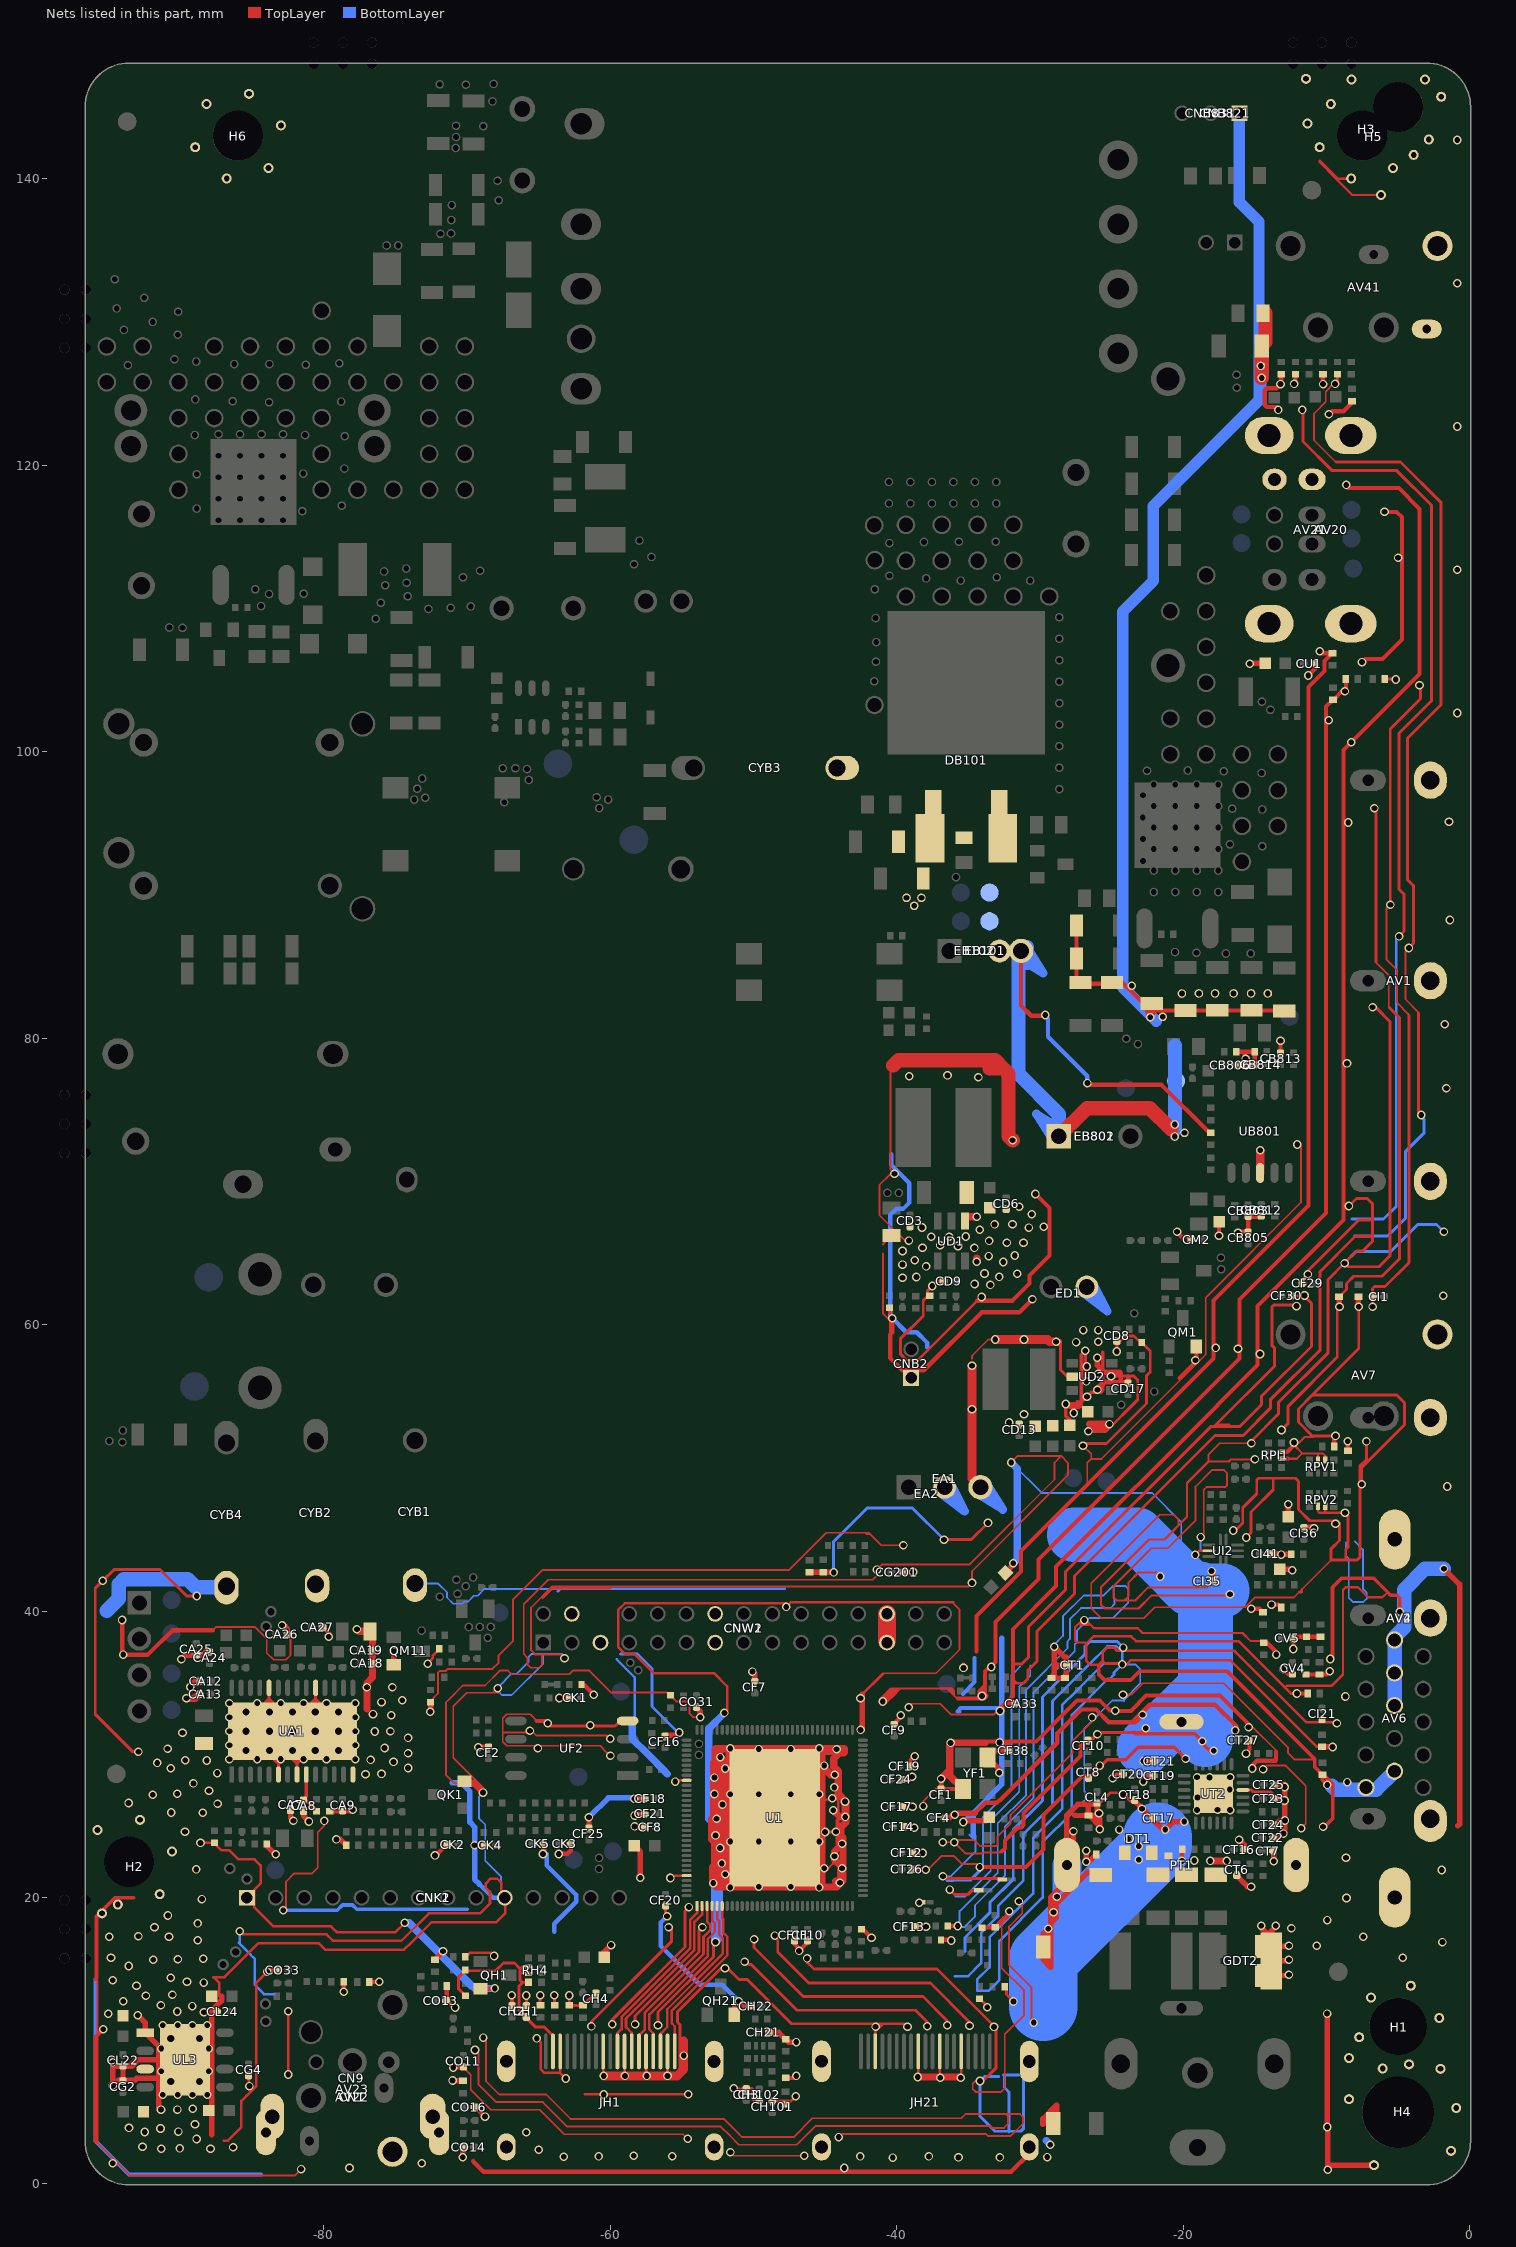
[diagram p0: the nets of this part, all layers, seen from the top]
# Altium PCB MISC86372.PcbDoc (part 10 of 16)
Units mm, origin at the board's own origin, x right, y up, seen from the top; angles counter-clockwise.
Board outline 96.73 x 148.13 mm, 2 copper layers (TopLayer, BottomLayer), stack 1.571 mm thick; 578 components, 318 nets, 2702 pads, 836 vias.

## Via types
v1: diameter 0.6, hole 0.4, TopLayer to BottomLayer, tented both sides, 816 vias
v2: diameter 0.7, hole 0.5, TopLayer to BottomLayer, tented both sides, 15 vias
v3: diameter 0.8, hole 0.5, TopLayer to BottomLayer, tented both sides, 5 vias

## Nets (pads, with @x,y where several pads share a name; then routed paths per layer and width w, separated by ;. In a path a pad name is that pad's centre, name@x,y a point inside that pad or via, vN(x,y) a via of type N, cw(c..) or ccw(c..) an arc to the next point about the centre after c; other vN are vias at no path point) (continued)
GND: (continued)
  TopLayer w0.381: CL22.2@-94.018,8.215 -94.018,7.235 CG2.1@-94.027,7.227 ; v1(-92.989,11.786) -92.471,11.267 UL3.1@-92.471,10.565 -91.535,9.628 -91.535,9.068 ; v1(-91.362,5.193) -91.535,5.365 -91.535,9.068 ; v1(-91.342,9.451) -91.535,9.258 -91.535,9.068 ; v1(-89.941,36.636) -89.664,36.913 -88.519,36.913 -88.255,37.176 CA24.1@-87.979,37.176 ; -87.817,3.445 -87.817,12.148 -87.252,12.713 -87.227,12.713 -87.114,12.826 -87.114,13.106 ; RA9.1@-83.972,23.724 -83.972,23.665 RA9.1@-83.917,23.61 ; RA9.1@-83.956,23.606 v1(-83.363,23.012) ; RA9.1@-83.917,23.568 RA9.1@-83.917,23.61 ; RA9.1@-83.917,23.728 RA9.1@-83.917,23.61 ; CA7.1@-82.324,26.043 -82.324,25.569 v1(-82.12,25.366) ; CA8.1@-81.417,25.981 -81.417,25.685 v1(-81.04,25.309) ; v1(-79.121,24.054) -78.841,24.054 DK1.A@-78.435,23.648 ; v1(-75.133,37.177) -75.108,37.151 QM11.E@-75.108,36.258 ; v1(-72.563,32.959) -72.542,32.98 RM12.2@-72.542,33.636 ; DO1.A@-72.238,15.665 -71.681,16.222 v1(-71.681,16.248) ; v1(-71.011,7.225) -70.979,7.193 DI8.A@-70.275,7.193 ; CO14.1@-70.312,2.577 -70.312,1.87 v1(-70.307,1.865) ; v1(-69.472,23.64) -69.462,23.63 CK4.2@-68.795,23.63 ; v1(-64.694,23.038) -64.631,23.1 CK5.2@-64.631,23.752 ; v1(-63.551,33.925) -63.535,33.941 CK1.1@-62.864,33.941 ; v1(-61.493,25.603) -61.487,25.597 CF25.2@-61.487,24.86 ; CF5.1@-60.406,15.824 -60.406,16.213 v1(-59.943,16.677) ; CF3.1@-58.321,23.628 -57.906,23.213 v1(-57.906,21.387) ; v1@-58.318,25.806 -57.651,25.806 CF21.2@-57.626,25.832 ; v1(-58.318,26.899) v1(-58.318,26.899) CF18.2@-57.634,26.898 ; v1@-58.318,26.924 -58.317,26.923 CF18.2@-57.634,26.923 ; -57.949,24.964 v1(-58.304,24.964) -58.28,24.94 CF8.1@-57.627,24.94 ; CF16.1@-56.185,31.286 -56.144,31.326 -55.389,31.326 v1(-55.194,31.521) ; CO31.1@-53.975,33.256 -53.722,33.002 v1(-53.722,32.578) ; v1(-50.076,35.773) -49.911,35.608 CF7.1@-49.911,35.096 ; CH21.2@-48.888,10.59 -48.24,10.59 DH23.A@-47.752,10.102 -47.556,9.906 v1(-47.015,9.906) ; CD101.A@-46.096,42.695 -45.156,42.695 CD102.A@-45.131,42.72 -44.428,42.72 v1(-44.403,42.696) ; v1(-42.524,31.699) -42.425,31.798 -42.425,33.807 v1(-42.534,33.916) -42.425,34.026 v1@-42.425,34.181 ; CF24.2@-39.605,28.245 -39.106,28.245 v1(-38.928,28.422) ; CG201.2@-39.58,42.723 v1@-38.862,42.723 ; CF14.1@-39.451,24.942 -38.843,24.942 v1(-38.773,24.872) ; CF13.1@-38.69,17.975 -37.985,17.975 v1(-37.959,17.95) ; CF4.1@-36.634,25.552 -36.304,25.552 ; CF4.1@-36.532,25.552 -36.304,25.552 ; v1(-35.956,25.786) v1@-36.07,25.786 ; v1@-35.325,25.241 v1(-35.357,25.273) -35.287,25.343 -33.802,25.343 CL3.1@-33.55,25.595 ; -34.533,25.895 -35.745,25.895 -35.855,25.786 v1@-36.07,25.786 ; YF1.4@-33.669,29.548 YF1.4@-33.669,29.777 ; v1@-32.919,28.778 v1(-32.842,28.702) -32.842,28.95 YF1.4@-33.669,29.777 ; CF15.1@-32.419,42.663 -31.877,43.205 v1(-31.877,43.332) ; -32.258,30.848 -32.258,30.391 -32.398,30.251 -33.194,30.251 YF1.4@-33.669,29.777 ; -29.413,15.596 CT47.1@-29.77,15.953 ; CT48.1@-29.084,4.208 -28.846,4.446 -28.846,5.498 -29.803,4.541 -29.803,4.166 -28.999,4.97 -28.999,5.135 ; -29.061,18.658 v1(-29.061,18.975) ; -29.007,36.22 CT1.2@-28.162,36.22 ; v1@-28.854,20.066 -29.061,19.859 -29.061,19.82 ; v1(-28.821,20.06) -29.061,19.82 ; -28.162,36.666 v1(-28.999,37.503) -29.007,37.495 -29.007,35.528 DK3.A@-29.21,35.325 DK2.A@-28.245,35.325 -28.162,35.407 -28.162,36.767 ; v1(-27.666,24.621) -27.666,22.719 PT1.4@-28.117,22.268 ; -27.559,25.756 -27.527,25.723 LT3.2@-26.619,25.723 ; v1(-26.764,23.256) v1(-26.764,22.498) -26.593,22.498 LT2.2@-26.079,23.012 ; -26.715,21.768 -26.715,21.721 -28.853,19.582 -28.853,18.593 -29.261,18.185 ; -26.619,26.51 LT3.2@-26.619,25.723 ; LT3.2@-26.556,25.723 -25.832,24.999 v1(-25.832,24.765) ; v1(-26.008,57.678) -26.008,57.162 -25.619,56.772 -25.522,56.675 -24.436,56.675 ; v1@-25.99,55.488 -25.99,55.542 -25.619,55.913 -25.522,56.01 ; CT18.2@-23.393,26.753 -22.885,26.245 v1(-22.885,26.187) -22.797,26.187 CT17.1@-22.142,25.532 -22.142,25.458 -21.423,24.74 -21.226,24.74 -20.667,25.298 v1(-19.939,25.298) ; DT1.3@-22.187,23.114 DT1.3@-22.187,23.177 ; CT6.1@-16.259,21.525 -16.259,21.49 -15.521,20.752 v1(-15.265,20.752) v1@-15.175,20.752 ; v1(-16.104,24.028) -15.704,23.629 CT16.2@-15.704,23.343 ; v1(-15.361,106.127) -15.335,106.153 CU2.2@-14.285,106.153 ; v1(-15.189,29.007) v1@-15.179,29.007 ; v1(-14.554,18.034) -14.554,17.856 -13.851,17.153 GDT2.2@-13.851,15.57 ; GDT2.2@-14.501,14.554 -12.675,14.554 v1(-12.624,14.605) ; GDT2.2@-14.501,16.586 -12.675,16.586 v1(-12.624,16.637) ; CI41.1@-13.85,43.993 v1@-13.208,43.993 ; CT7.1@-13.692,23.341 -13.692,22.607 v1@-13.691,22.606 ; CT22.2@-13.692,24.154 -13.336,24.154 v1@-13.03,24.46 ; CT23.1@-13.625,26.928 -12.933,26.928 v1@-12.929,26.924 ; CT25.2@-13.596,27.864 -13.066,27.864 v1(-12.918,27.716) ; CT25.2@-13.596,27.915 v1@-12.907,27.915 ; v1(-13.538,18.034) -13.538,17.958 -13.851,17.644 GDT2.2@-13.851,15.57 ; CI40.1@-13.264,42.901 -12.446,42.901 v1(-12.395,42.85) ; v1(-13.157,43.942) v1@-13.208,43.993 ; v1(-13.005,24.46) v1@-13.03,24.46 ; -12.903,27.407 v1(-12.903,25.375) -12.903,24.587 v1@-13.03,24.46 ; CI9.1@-12.675,46.579 v1(-12.675,47.447) ; v1(-12.624,15.646) -12.7,15.57 GDT2.2@-13.851,15.57 ; RI43.1@-12.465,43.967 -13.183,43.967 v1@-13.208,43.993 ; CI36.1@-11.582,45.84 -10.94,45.84 v1(-10.871,45.771) ; DV5.A@-10.312,30.512 -9.583,30.512 v1(-9.576,30.505) ; v1(-9.957,11.898) -9.946,11.887 v1(-9.946,3.978) -9.919,3.951 v1(-9.919,0.991) -9.598,1.311 H4.3@-6.678,1.311 ; DI2.A@-9.119,61.932 -9.119,61.265 v1(-9.093,61.239) ; DI3.A@-7.772,61.932 -7.772,61.265 v1(-7.747,61.239) ; v1(-1.803,42.946) -0.711,41.853 -0.711,25.129 -0.838,25.002 ; CG2.1@-94.027,7.227 -94.367,7.227 v1(-94.721,6.873) v1(-94.721,8.487) -94.447,8.213 -93.39,8.213 ; CG2.1@-94.027,7.227 -93.192,7.227 -93.046,7.372 -90.976,7.372 UL3.EPAD@-89.689,8.66 -89.706,8.677 -92.71,8.677 ; -93.39,8.213 -92.925,8.677 -92.71,8.677 ; -93.39,8.213 -93.406,8.23 -93.574,8.23 -93.126,8.677 -92.71,8.677 ; -36.304,25.552 v1@-36.07,25.786 ; CT47.1@-29.77,15.953 CT47.1@-29.77,16.561 ; CT47.1@-29.77,15.953 -29.77,15.637 -29.261,15.127 v1@-29.261,17.984 ; CT47.1@-29.77,16.561 -29.431,16.9 v1(-29.431,17.813) ; CT47.1@-29.77,16.561 -29.77,17.474 v1(-29.431,17.813) ; v1(-29.431,17.813) v1@-29.261,17.984 ; v1@-29.261,17.984 -29.261,18.185 ; -29.261,18.185 v1@-29.261,19.175 ; v1@-29.261,19.175 v1(-29.061,18.975) ; v1@-29.261,19.175 -29.261,20.009 -28.117,21.153 PT1.4@-28.117,22.268 ; v1(-29.061,18.975) -29.061,19.82 ; PT1.4@-28.117,22.268 -28.117,25.757 -27.364,26.51 -26.063,26.51 CL4.1@-26.01,26.563 -26.01,26.01 v1(-25.883,25.883) ; LT3.2@-26.619,25.723 v1@-26.042,25.723 ; v1@-26.042,25.723 v1(-25.883,25.883) ; v1@-26.042,25.723 -25.832,25.514 v1(-25.832,24.765) ; v1(-25.883,25.883) -25.883,24.816 v1(-25.832,24.765)
  TopLayer w0.508: v1(-89.586,33.909) -88.972,33.909 CA13.1@-88.693,34.188 ; v1(-89.332,34.696) -88.923,35.105 CA12.1@-88.668,35.105 ; v1(-77.686,38.73) -77.538,38.583 CA2.1@-76.733,38.583 ; -76.987,33.172 v1(-76.987,34.671) -76.987,34.98 -76.6,35.367 CA19.1@-76.6,37.272 -76.6,38.49 CA2.1@-76.811,38.701 ; QK1.E@-70.053,27.978 -69.472,27.978 -68.883,27.388 v1(-68.883,27.323) ; v1(-52.654,24.333) v1@-52.654,24.319 ; v1(-52.578,25.502) -52.511,25.569 -52.511,29.227 -52.368,29.369 -52.368,30.164 -52.138,30.393 ; v1@-52.553,24.511 -52.393,24.352 -52.393,24.058 ; v1@-52.485,25.649 -52.612,25.522 v1@-52.612,24.277 ; -52.451,26.873 v1@-52.451,27.178 ; v1(-52.333,23.457) v1@-52.393,23.518 ; v1(-52.322,29.805) -52.172,29.655 v1@-52.172,26.67 ; -52.307,20.735 -52.473,20.9 -52.473,21.357 ; v1(-52.222,22.377) -52.222,21.59 -52.121,21.488 -52.341,21.488 ; -52.063,23.727 -52.172,23.836 ; -51.968,21.099 -51.85,20.98 -51.689,20.98 -51.713,21.005 -51.713,21.96 -51.713,22.719 -51.713,25.556 -51.713,26.406 -51.713,30.299 -51.816,30.402 v1@-45.237,30.402 ; -51.663,28.056 -52.414,28.056 v1(-52.73,28.372) v1(-52.73,27.229) v1@-52.172,26.67 ; -50.317,30.402 -50.326,30.393 -52.138,30.393 ; v1@-45.313,30.206 -44.351,30.206 v1(-44.201,30.356) ; v1(-45.06,29.21) -45.231,29.21 v1@-45.237,29.204 ; v1(-44.425,26.086) -43.963,25.624 v1(-43.597,25.624) -43.612,25.639 v1(-43.612,26.695) -43.612,26.766 -44.084,27.238 ; v1(-44.323,28.575) -44.609,28.575 v1@-45.237,29.204 ; -44.27,21.125 v1@-43.786,21.125 ; v1(-43.967,21.031) -43.915,21.084 -43.915,21.948 v1(-43.815,22.047) -43.815,22.108 -44.348,22.642 v1(-44.348,22.885) -44.348,23.216 v1(-43.815,23.749) -43.912,23.846 -43.912,24.331 ; v1(-38.532,7.468) -37,7.468 -35.567,7.468 v1@-35.5,7.401 ; v1(-36.906,28.296) -36.3,28.902 -36.3,29.896 ; v1(-36.241,30.794) -36.3,30.735 -36.3,29.896 ; YF1.2@-35.369,27.577 -36.3,28.508 -36.3,29.896 ; -34.855,67.52 v1(-34.421,67.52) ; v1(-34.41,64.38) v1@-34.41,64.644 ; v1@-18.11,22.544 v1(-18.11,22.555) v1(-16.967,22.555) ; v1@-52.654,24.319 v1@-52.612,24.277 ; v1@-52.654,24.319 -52.654,23.778 v1@-52.393,23.518 ; v1@-52.612,24.277 -52.393,24.058 ; v1@-52.612,24.277 -52.612,24.079 -52.393,23.86 v1@-52.393,23.518 ; -52.473,21.357 -52.341,21.488 ; -52.473,21.357 -52.473,21.381 -52.473,23.216 -52.393,23.296 v1@-52.393,23.518 ; -52.393,24.058 -52.172,23.836 ; -52.341,21.488 -52.172,21.658 -52.172,21.682 -52.172,23.836 ; -52.172,23.836 v1(-52.172,26.492) v1@-52.172,26.67 ; -52.138,30.393 -52.649,30.393 -52.673,30.37 -52.673,29.483 -52.79,29.365 -52.79,25.606 -52.917,25.479 -52.917,24.068 -52.698,23.85 -52.698,22.295 -52.866,22.127 -52.866,20.988 -52.614,20.735 v1@-45.187,20.735 ; v1@-45.237,29.204 v1@-45.237,30.402 ; v1@-45.237,29.204 -45.237,20.786 v1@-45.187,20.735 ; v1@-45.237,30.402 -43.652,30.402 -43.652,30.119 -43.677,30.094 -43.995,30.094 -44.323,29.767 -44.394,29.695 -44.394,29.131 -44.323,29.06 -44.084,28.821 -44.084,27.238 ; v1@-45.187,20.735 -44.176,20.735 v1@-43.786,21.125 ; -44.084,27.238 -43.551,26.705 -43.551,25.256 -43.912,24.895 -43.912,24.331 ; -43.912,24.331 -43.754,24.173 -43.754,21.157 v1@-43.786,21.125 ; v1(-40.97,33.68) -40.97,33.783 -40.35,34.404 -40.164,34.404 -40.887,33.68 v1(-40.97,33.68) ; -26.534,53.051 v1(-25.155,53.051) -25.425,52.781 -26.264,52.781 -26.534,53.051
  TopLayer w0.6: DB101.1@-37.49,92.837 DB101.1@-37.49,93.116 ; UB801.3@-14.63,70.582 v1(-14.63,72.161)
  TopLayer w0.61: v1(-60.452,7.544) v1(-58.979,7.544) v1(-57.455,7.544) v1(-56.007,7.544) ; v1@-56,7.551 -55.993,7.544 -55.335,7.544 -54.868,8.011 v1(-54.868,8.966) -54.868,9.979 ; v1(-34.748,57.125) v1(-34.748,54.077) -34.748,49.233 EA1.2@-34.158,48.643 ; v1(-33.122,58.953) v1(-31.115,58.953) -29.461,58.953 -29.308,58.801 v1(-28.88,58.801)
  TopLayer w0.8: -22.271,81.918 -22.25,81.939
  TopLayer w1: -40.244,78.078 -39.874,78.448 -33.132,78.448 -32.554,77.87 ; -33.519,77.87 -32.554,77.87 ; v1(-31.913,72.874) -32.194,73.155 -32.194,77.51 -32.554,77.87 ; EB801.1@-28.687,73.139 -26.719,75.108 -22.33,75.108 -20.834,73.612 ; pad.VIA5@-14.527,126.087 CB808.1@-14.527,128.322 -14.259,128.59 RB847.1@-14.259,130.607
  TopLayer w1.27: CNW2.25@-40.681,37.897 CNW2.26@-40.681,39.796
  BottomLayer w0.127: CYB1.2@-73.635,41.914 -72.013,41.914 -71.399,41.3 -71.399,40.945 -70.968,40.513 -70.349,40.513 -70.196,40.665 -69.93,40.665 -69.53,41.065 -69.263,41.065 -68.792,41.537 -63.491,41.537 -63.422,41.537 ; v1(-68.883,27.323) -69.171,27.035 -69.171,25.537 -68.728,25.094 -68.728,22.552 -67.623,21.446 ; -67.642,21.466 -67.623,21.446 ; CNK2.10@-67.623,20.248 -67.623,21.446 ; -63.373,36.996 -64.694,36.996 ; -35.916,20.066 -35.255,20.066 -33.439,21.882 -33.439,25.404 -31.453,27.39 -31.453,34.714 -30.683,35.484 -30.683,36.195 ; v1@-35.611,17.958 -35.611,19.055 -32.948,21.718 -32.948,25.172 -30.97,27.15 -30.97,34.505 -28.08,37.396 -28.08,37.891 -27.915,38.056 -27.915,39.424 -27.139,40.2 -25.131,40.2 ; -35.441,17.951 -35.262,17.951 -34.544,18.669 -34.544,19.439 -32.44,21.544 ; -34.946,24.389 -34.506,23.949 ; -34.658,24.308 -34.709,24.359 -34.823,24.359 -34.506,24.041 -34.506,23.949 ; -34.658,24.502 -34.506,24.35 -34.506,23.949 ; -32.44,21.717 -32.44,21.544 ; v1(-32.007,50.368) -29.886,48.247 -22.18,48.247 -20.142,46.21 -20.142,43.92 -20.989,43.073 ; -31.394,36.116 -31.986,35.524 -31.986,27.611 -33.972,25.625 -33.972,22.031 -34.808,21.196 -36.487,21.196 v1(-36.779,21.488) -36.22,21.488 -34.506,23.203 -34.506,23.949 ; v1@-28.931,37.723 -28.397,38.256 -28.397,39.624 -26.928,41.093 -25.595,41.093 ; -27.78,25.907 -26.815,26.873 -26.815,27.32 -26.913,27.418 -26.913,31.783 -24.94,33.757 -24.192,33.757 -24.13,33.819 ; -25.544,41.093 -24.879,41.758 -24.816,41.758 ; -25.08,40.2 -24.808,40.473 -24.808,40.861 -24.849,40.902 -24.849,41.724 -24.816,41.758 ; -24.942,39.522 -26.546,39.522 -27.407,38.662 -27.407,37.846 -27.572,37.681 -27.572,37.185 -30.462,34.295 -30.462,26.939 -30.611,26.791 -32.44,24.962 -32.44,21.544 ; -24.891,39.522 -23.84,40.573 -23.84,41.536 -24.061,41.758 -24.816,41.758 ; v1(-24.257,36.271) -23.341,36.271 -23,35.93 -23,34.949 -24.13,33.819 ; -24.13,33.706 -24.13,33.819 ; v1(-19.156,43.917) -18.796,44.276 v1@-18.796,45.161 ; -8.644,44.78 -8.644,43.866 -8.445,43.667 -8.445,40.934 -8.152,40.64 -7.416,40.64 -7.188,40.869 -7.188,41.278 -7.458,41.547 -7.458,44.288 -8.026,44.856 ; v1(-4.877,39.954) v1@-4.877,40.005 ; -64.694,36.996 -65.516,36.996 -65.692,36.819 -65.692,36.461 -66.542,35.611 -66.904,35.611 -67.766,34.748 -67.766,34.339 -67.565,34.138 -66.883,34.138 -64.694,36.327 -64.694,36.996
  BottomLayer w0.178: -85.948,16.84 -85.113,16.005 ; v1(-85.87,17.644) -85.87,16.774 -85.113,16.017 -85.113,16.005 ; -83.472,13.259 -84.176,13.259 -84.836,13.919 -84.836,15.728 -85.113,16.005 ; v1(-74.346,18.237) -69.763,13.654 v1(-68.062,13.654) ; -63.658,41.37 -63.491,41.537 -63.466,41.562 -47.836,41.562 ; -59.563,36.635 -58.293,35.365 -58.293,31.136 -57.275,30.117 ; -57.573,30.117 -57.508,30.117 -57.275,30.117 ; -56.019,28.629 -56.019,28.862 -57.275,30.117 ; -35.941,14.503 -35.021,14.503 -34.112,15.412 -34.112,17.517 -32.929,18.7 -32.929,19.403 -31.16,21.172 -31.16,24.432 -29.126,26.465 -29.126,33.711 -26.669,36.168 -25.296,37.541 -24.663,37.541 -24.257,37.135 v1(-24.257,36.271) ; v1(-24.257,36.271) -24.321,36.335 -25.55,36.335 -26.912,34.973 -27.488,34.397 -28.453,33.432 -28.453,26.186 -30.487,24.153 -30.487,20.271 -33.506,17.252 -33.506,15.161 -34.366,14.301 -34.366,13.487 -33.604,13.487 -32.842,14.249 -32.842,16.964 -29.813,19.993 -29.813,23.874 -27.78,25.907 -27.78,32.748 -25.255,35.273 -25.121,35.273 -24.833,35.56 -24.833,35.695 v1(-24.257,36.271)
  BottomLayer w0.203: -59.284,37.008 -58.109,37.008 -57.087,35.986 -57.087,33.337 v1@-55.232,31.483 ; v1(-44.403,42.696) -44.403,44.851 -42.059,47.196 -38.915,47.196 v1(-36.703,44.983) ; -36.487,21.196 -36.068,21.196 -36.005,21.259 -34.834,21.259 -34.215,21.879 v1(-34.215,22.123) ; -35.23,16.231 -35.23,17.211 -33.503,18.938 -33.503,19.641 -31.868,21.275 -31.868,24.725 -29.835,26.759 -29.835,34.004 ; -32.88,7.51 -33.867,7.51 v1(-34.188,7.188) -34.188,4.731 -33.141,3.683 -32.156,3.683 ; -32.156,3.632 -32.156,3.683 ; -31.481,7.62 -32.543,7.62 -32.487,7.564 -32.487,6.733 -32.156,6.403 -32.156,3.683 ; JH21.22@-30.75,8.55 -31.138,8.162 -31.138,3.889 -31.344,3.683 -32.156,3.683 ; -27.17,36.669 -28.502,35.337 ; v1(-24.18,37.447) -24.618,37.885 -26.515,37.885 -26.848,37.552 -26.848,36.991 -28.502,35.337 ; v1(-8.738,64.287) -7.915,65.11 -5.496,65.11 -3.626,66.98 -2.311,66.98 v1(-1.803,66.472) ; -8.23,67.361 -6.021,67.361 -5.131,68.251 ; -8.052,66.192 -5.715,66.192 -4.47,67.437 ; -5.131,68.783 -5.131,68.251 ; v1(-4.932,87.096) -5.131,86.898 -5.131,68.251 ; -4.47,68.148 -4.47,67.437 ; v1(-3.378,74.625) -3.378,74.524 -3.18,74.325 -3.18,73.382 -4.47,72.092 -4.47,67.437 ; -29.835,34.004 -28.502,35.337 ; -29.835,34.004 -28.502,35.337
  BottomLayer w0.254: -95.94,14.301 -95.94,3 -93.6,0.66 -84.387,0.66 ; v1@-82.751,19.186 v1(-82.828,19.109) -79.056,19.109 -78.687,19.477 -77.989,19.477 -77.698,19.186 -70.002,19.186
  BottomLayer w0.279: -35.636,33.002 -35.762,33.002 -35.536,33.229 v1@-32.756,33.229 ; -35.386,34.214 -34.566,35.033 -34.566,36.709
  BottomLayer w0.3: EB101.2@-31.504,85.899 EB101.2@-31.323,86.081 ; v1@-29.642,81.559 -29.439,81.356 -29.439,80.086 -28.258,78.905 ; -27.203,77.851 -28.258,78.905 ; v1(-26.692,76.857) -26.692,77.339 -28.258,78.905
  BottomLayer w0.305: -69.335,21.133 -68.192,19.99 CNK2.10@-67.365,19.99 ; v1@-64.44,23.038 -64.44,22.238 -62.382,20.181 -62.382,19.695 -63.906,18.171 -63.906,17.602 ; v1(-56.032,18.694) -56.469,18.258 -56.469,16.616 -53.759,13.906 -52.176,13.906 v1(-51.033,12.763) ; -40.386,71.89 -40.386,71.14 -39.116,69.87 -39.116,68.521 -39.565,68.072 -40.03,68.072 -40.464,67.639 -40.464,60.595 v1(-40.316,60.448) -39.33,59.461 -38.606,59.461 -37.882,58.737 -37.882,58.395
  BottomLayer w0.381: -71.044,28.016 -70.438,28.016 -69.806,27.384 -69.806,25.255 -69.472,24.922 -69.472,21.271 -69.132,20.93 ; v1(-61.493,25.603) -60.139,26.957 v1@-58.438,26.957 ; v1(-35.357,25.273) -35.294,25.273 -34.658,25.909 ; -34.658,24.308 -34.658,24.502 -34.658,25.909 ; -32.672,38.108 -32.672,27.895 -34.658,25.909
  BottomLayer w0.508: v1(-74.346,18.237) -74.041,18.237 -69.457,13.654 v1(-68.062,13.654) ; -58.458,31.944 -58.458,31.067 -57.508,30.117 -56.019,28.629 ; v1@-55.85,21.407 v1(-55.804,21.361) ; v1(-52.03,32.887) -53.13,31.786 -53.13,30.56 -53.137,30.553 -53.137,30.37 -53.13,30.363 -53.13,29.792 -53.137,29.785 -53.137,25.756 ; v1(-32.007,50.368) -31.593,49.954 -31.593,43.617 v1(-31.877,43.332) ; -29.57,3.032 v1(-29.286,2.748) ; -53.137,25.756 -53.137,25.476 -52.698,25.037 ; -53.137,25.756 -52.698,25.317 -52.698,25.037 ; -52.698,25.037 -52.698,16.935 v1(-52.654,16.891) -52.393,17.152 -52.393,24.733 -52.698,25.037
  BottomLayer w0.8: -21.869,81.178 -24.232,83.541 -24.232,109.779 -22.098,111.912 -22.098,117.145 -14.58,124.663 pad.VIA5@-14.58,126.924 ; CNB831.1@-16.081,144.562 -16.081,138.356 -14.712,136.988 -14.712,124.531
  BottomLayer w1: EB101.2@-31.504,85.899 -31.504,77.503 -28.687,74.687 EB801.1@-28.687,73.851 ; -30.903,85.235 -30.903,85.661 EB101.2@-30.903,86.343 ; EB801.1@-29.107,73.559 EB801.1@-28.687,73.139 ; -20.574,73.612 -20.574,79.477
  BottomLayer w1.016: -95.148,40.015 -94.312,40.851 -94.312,41.851 -93.955,42.209 -89.503,42.209 -88.951,41.656 -86.868,41.656 -86.741,41.529 CYB4.2@-86.883,41.387 ; -9.627,27.788 -9.359,27.52 -6.542,27.52 AV6.10@-5.247,28.815 ; AV6.8@-5.247,33.395 AV6.7@-5.247,35.685 AV6.6@-5.247,37.975 -5.247,38.196 -4.58,38.863 -4.58,41.496 -3.13,42.946 v1(-1.803,42.946)
  BottomLayer w2.032: v1@-29.638,17.607 -28.105,19.141 PT1.4@-28.105,22.256
  BottomLayer w3.81: -27.592,45.314 -23.23,45.314 -20.122,42.205 -20.122,42.118 -19.559,41.555 -18.839,41.555 -18.686,41.402 ; -22.733,30.429 -18.445,34.717 -18.445,36.17 ; v1@-18.445,31.006 -18.445,36.17 ; -17.265,41.402 -18.686,41.402 ; -18.686,41.402 -18.445,41.161 -18.445,36.17
  BottomLayer w4.8: -29.769,12.37 -29.769,15.691 -21.793,23.667 -21.793,24.232
  other v1: -78.207,1.118 -43.663,1.118 -94.742,1.448 -73.165,1.44 -40.278,1.841 -35.687,1.854 -32.798,1.854 -29.5,1.88 -63.256,1.905 -60.808,1.924 -55.677,1.945 -42.545,1.924 -37.754,1.924 -58.369,1.967 -64.999,2.388 -91.343,2.455 -87.909,2.464 -90.065,2.484 -86.335,2.565 -92.659,2.591 -88.881,3.141 -65.862,3.607 -92.507,3.632 -90.148,3.658 -91.397,3.875 -93.599,3.912 -88.992,4.172 -90.219,5.193 -89.144,5.244 -91.236,6.238 -90.205,6.238 -89.173,6.238 -88.141,6.238 -35.535,7.417 -91.342,7.869 -88.036,7.869 -88.036,9.451 -91.236,11.082 -90.205,11.082 -89.173,11.082 -88.141,11.082 -95.05,11.887 -88.361,11.989 -90.238,12.044 -89.193,12.421 -91.373,12.484 -94,12.751 -92.416,13.139 -90.568,13.211 -93.078,13.84 -88.377,14.062 -89.552,14.122 -94.739,14.232 -90.678,14.401 -93.61,15.215 -91.897,15.646 -90.182,15.697 -88.417,15.723 -94.857,15.785 -4.674,15.785 -10.685,16.637 -1.905,16.888 -88.798,17.018 -94.977,17.253 -90.804,17.253 -7.442,17.253 -92.944,17.287 -12.45,17.856 -91.821,17.932 -88.798,18.19 -9.942,18.425 -90.881,18.745 -32.156,19.034 -88.507,19.888 -8.601,19.964 -51.616,20.703 -45.41,20.703 -49.631,20.753 -47.396,20.753 -1.956,21.92 -88.9,21.96 -13.691,22.53 -19.228,22.581 -23.114,22.631 -8.636,22.781 -23.114,23.571 -51.616,23.905 -49.631,23.905 -47.396,23.905 -45.41,23.905 -23.851,24.105 -89.687,24.587 -24.46,24.74 -21.26,24.74 -58.303,25.722 -88.443,25.908 -90.653,25.933 -19.032,26.104 -16.732,26.104 -17.602,26.129 -87.417,26.54 -93.627,26.599 -12.929,26.772 -44.501,26.924 -19.007,26.974 -91.95,27.183 -51.616,27.207 -49.631,27.207 -47.396,27.207 -45.41,27.207 -90.227,27.246 -88.018,27.457 -16.757,27.534 -89.103,27.965 -8.544,28.055 -18.162,28.379 -19.032,28.404 -16.732,28.404 -77.089,28.6 -75.971,28.626 -87.437,28.686 -90.689,29.015 -74.117,29.043 -91.63,29.396 -75.133,29.465 -89.664,29.581 -88.163,29.566 -76.733,29.607 -86.59,29.658 -84.638,29.663 -83.013,29.663 -81.413,29.663 -79.813,29.663 -77.803,29.658 -74.117,30.07 -49.631,30.359 -47.396,30.359 -90.907,30.393 -51.616,30.409 -45.41,30.409 -75.754,30.434 -86.59,30.634 -77.803,30.634 -74.117,31.14 -89.865,31.496 -76.442,31.586 -86.59,31.611 -77.803,31.611 -75.35,31.611 -65.608,31.648 -86.59,32.588 -77.803,32.588 -75.292,32.725 -76.564,32.807 -86.59,33.565 -77.803,33.565 -84.638,33.57 -83.013,33.57 -81.413,33.57 -79.813,33.57 -75.971,33.644 -74.53,33.766 -8.678,34.032 -75.209,34.685 -26.903,39.365 -38.862,42.723 -1.565,48.694 -32.156,53.162 -31.115,53.73 -27.635,53.823 -25.933,56.56 -26.728,57.068 -24.638,58.115 -27.483,58.776 -25.931,58.799 -26.975,59.614 -25.933,59.614 -34.081,61.925 -1.854,62.001 -33.462,62.767 -34.569,62.831 -39.599,63.274 -38.629,63.318 -32.849,63.322 -33.872,63.563 -31.598,63.551 -37.954,64.059 -39.599,64.186 -32.563,64.367 -38.735,64.491 -33.579,64.781 -31.758,64.821 -39.599,65.136 -38.202,65.354 -34.579,65.347 -35.726,65.486 -36.976,65.53 -32.309,65.71 -31.151,65.718 -33.553,65.837 -39.151,65.863 -37.599,66.13 -36.347,66.13 -35.179,66.148 -34.203,66.624 -38.239,66.777 -30.776,66.77 -29.739,66.833 -33.172,66.991 -31.917,67.006 -30.578,67.695 -31.441,68.224 -1.626,76.505 -34.299,77.26 -39.125,77.336 -36.458,77.393 -8.568,78.228 -13.208,79.807 -1.742,80.957 -29.642,81.61 -1.382,88.24 -8.484,95.047 -1.448,95.098 -0.864,102.692 -0.864,112.692 -5.004,113.54 -0.864,122.692 -0.864,132.692 -0.864,142.692
  other v2: -85.423,30.261 -83.797,30.261 -82.197,30.261 -80.597,30.261 -78.971,30.261 -85.423,31.611 -83.797,31.611 -82.197,31.611 -80.597,31.611 -78.971,31.611 -85.423,32.961 -83.797,32.961 -82.197,32.961 -80.597,32.961 -78.971,32.961
  other v3: -90.689,7.16 -88.689,7.16 -90.689,10.16 -88.689,10.16
GND1: H6.1 H6.2 H6.3 H6.4 H6.5 H6.6
GVDD: CA8.2@-81.417,26.656 CA8.2@-81.417,26.831 RA10.1 UA1.9 | length 3.1
  TopLayer w0.254: UA1.9@-81.222,28.611 -81.222,27.026 CA8.2@-81.417,26.831 -81.258,26.831 RA10.1@-80.502,26.075
HDMI_A_0N_IN_IC: JH1.9 U1.1 | length 12.6
  TopLayer w0.178: JH1.9@-59.5,9.258 -59.5,10.528 -59.207,10.82 -59.207,11.671 -54.432,16.446 -54.432,18.414 -53.938,18.908 U1.1@-53.938,19.506
HDMI_A_0P_IN_IC: JH1.7 U1.2 | length 12.5
  TopLayer w0.178: JH1.7@-58.5,9.258 -58.5,10.545 -58.903,10.947 -58.903,11.545 -54.127,16.32 -54.127,18.288 -53.588,18.827 U1.2@-53.588,19.406
HDMI_A_1N_IN_IC: JH1.6 U1.3 | length 12.3
  TopLayer w0.178: JH1.6@-58,9.258 -58,10.377 -57.582,10.795 -57.582,11.968 -53.492,16.057 -53.492,17.247 -53.012,17.727 -53.012,18.093 -53.238,18.319 U1.3@-53.238,19.406
HDMI_A_1P_IN_IC: JH1.4 U1.4 | length 12.2
  TopLayer w0.178: JH1.4@-57,9.258 -57,10.518 -57.277,10.795 -57.277,11.841 -53.188,15.931 -53.188,17.12 -52.707,17.6 -52.707,18.219 -52.888,18.4 U1.4@-52.888,19.406
HDMI_A_2N_IN_IC: JH1.3 U1.5 | length 12.1
  TopLayer w0.178: JH1.3@-56.5,9.258 -56.5,10.48 -56.023,10.957 -56.023,12.198 -52.138,16.082 -52.138,17.138 -52.403,17.402 -52.403,18.365 -52.538,18.501 U1.5@-52.538,19.406
HDMI_A_2P_IN_IC: JH1.1 U1.6 | length 12
  TopLayer w0.178: JH1.1@-55.5,9.258 -55.5,11.011 -55.718,11.229 -55.718,12.071 -51.834,15.956 -51.834,17.264 -52.098,17.528 -52.098,18.492 -52.188,18.582 U1.6@-52.188,19.406
HDMI_A_5V: CH1.1 JH1.18 RH3.2 RH4.3 RH4.5 RH4.7 RH81.2 | length 15.6
  TopLayer w0.203: RH81.2@-70.111,14.884 -68,14.884 -67.465,15.42 -66.696,15.42 -66.359,15.083 -66.191,15.083 ; RH81.2@-70.111,14.935 -70.583,14.463 -70.583,13.617 RH3.2@-70.104,13.139 ; CH1.1@-65.862,11.619 -66.365,12.122 -66.365,13.81 -66.09,14.085 ; CH1.1@-65.862,11.794 -65.862,11.608 -65.202,10.947 -64.599,10.947 -64,10.349 JH1.18@-64,9.258 ; RH4.7@-65.703,14.085 -66.09,14.085 ; RH4.5@-65.703,14.685 -66.294,14.685 ; RH4.3@-65.703,15.185 -66.089,15.185 -66.191,15.083 ; -66.294,14.685 -66.294,14.98 -66.191,15.083 ; -66.294,14.685 -66.294,14.221 -66.158,14.085 -66.09,14.085